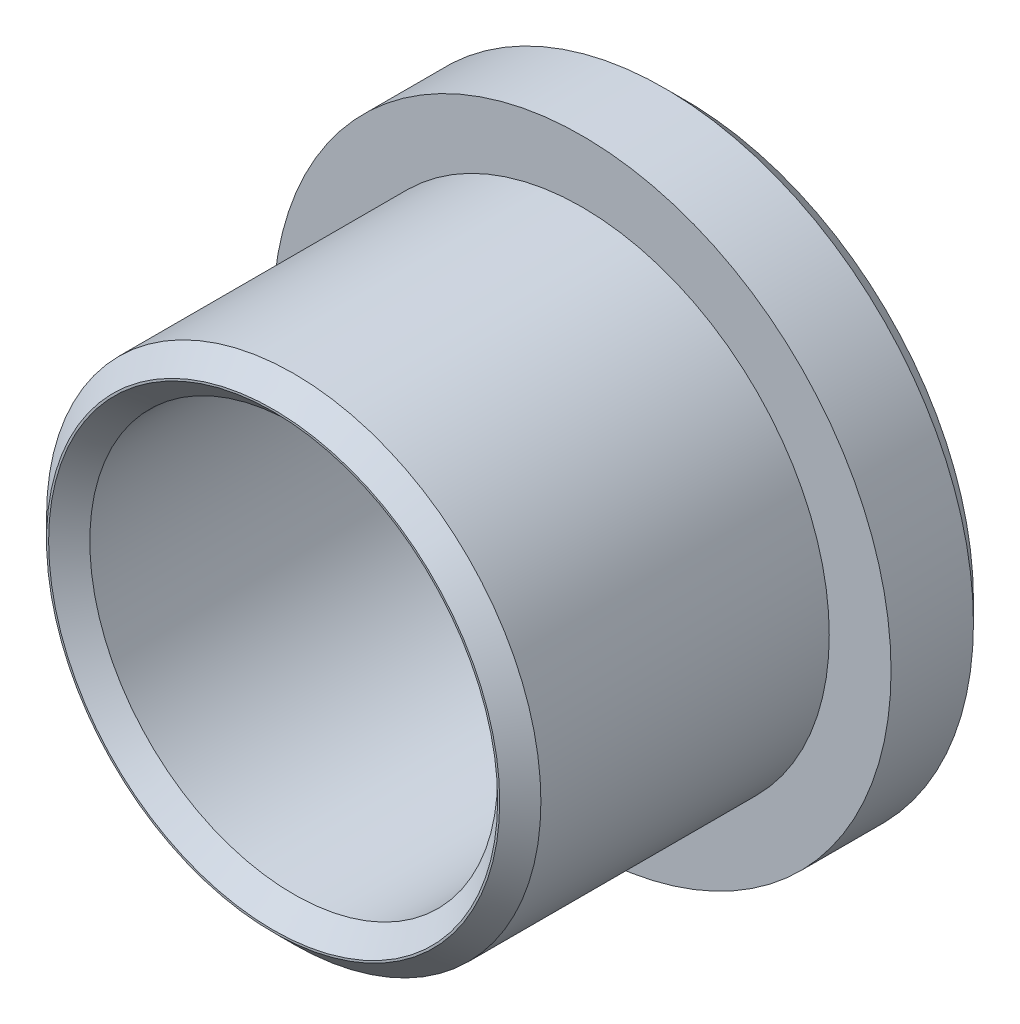
from build123d import *

# Parameters (mm, degrees)
SKETCH1_R           = 15
SKETCH1_R_2         = 9.9
BOSS_EXTRUDE1_DEPTH = 5
SKETCH2_R           = 12
SKETCH2_R_2         = 9.9
BOSS_EXTRUDE2_DEPTH = 15
CHAMFER1_SIZE       = 1


with BuildPart() as part:
    # Sketch1 → Boss-Extrude1 (new body)
    with BuildSketch(Plane.XY):
        Circle(SKETCH1_R)
        Circle(SKETCH1_R_2, mode=Mode.SUBTRACT)
    extrude(amount=BOSS_EXTRUDE1_DEPTH)

    # Sketch2 → Boss-Extrude2 (add)
    with BuildSketch(Plane.XY.offset(5)):
        Circle(SKETCH2_R)
        Circle(SKETCH2_R_2, mode=Mode.SUBTRACT)
    extrude(amount=BOSS_EXTRUDE2_DEPTH)

    # Chamfer1
    chamfer1_edges = [part.edges().sort_by_distance(p)[0] for p in [
        (-12, 0, 20),
        (-9.9, 0, 20),
        (-15, 0, 0),
    ]]
    chamfer(chamfer1_edges, length=CHAMFER1_SIZE)


solid = part.part
